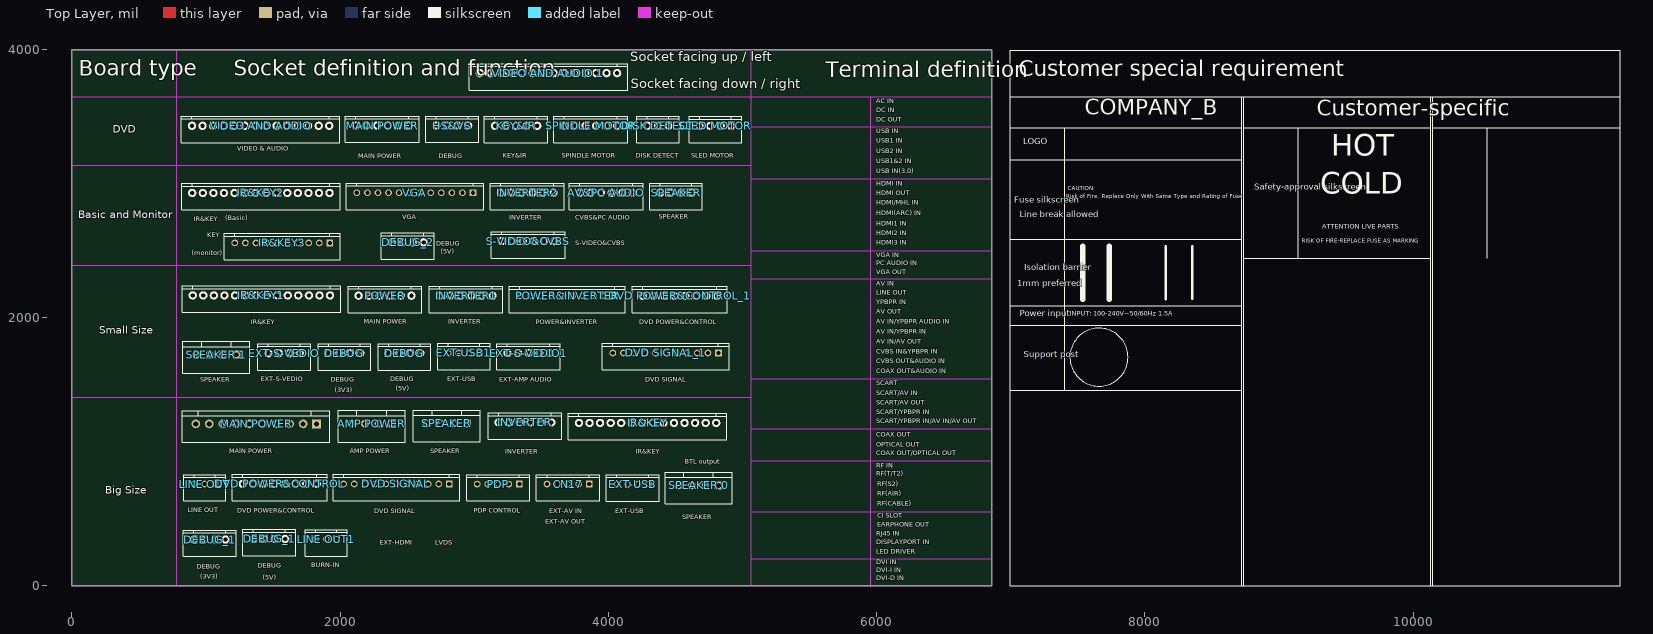
[diagram p0: Top Layer view]
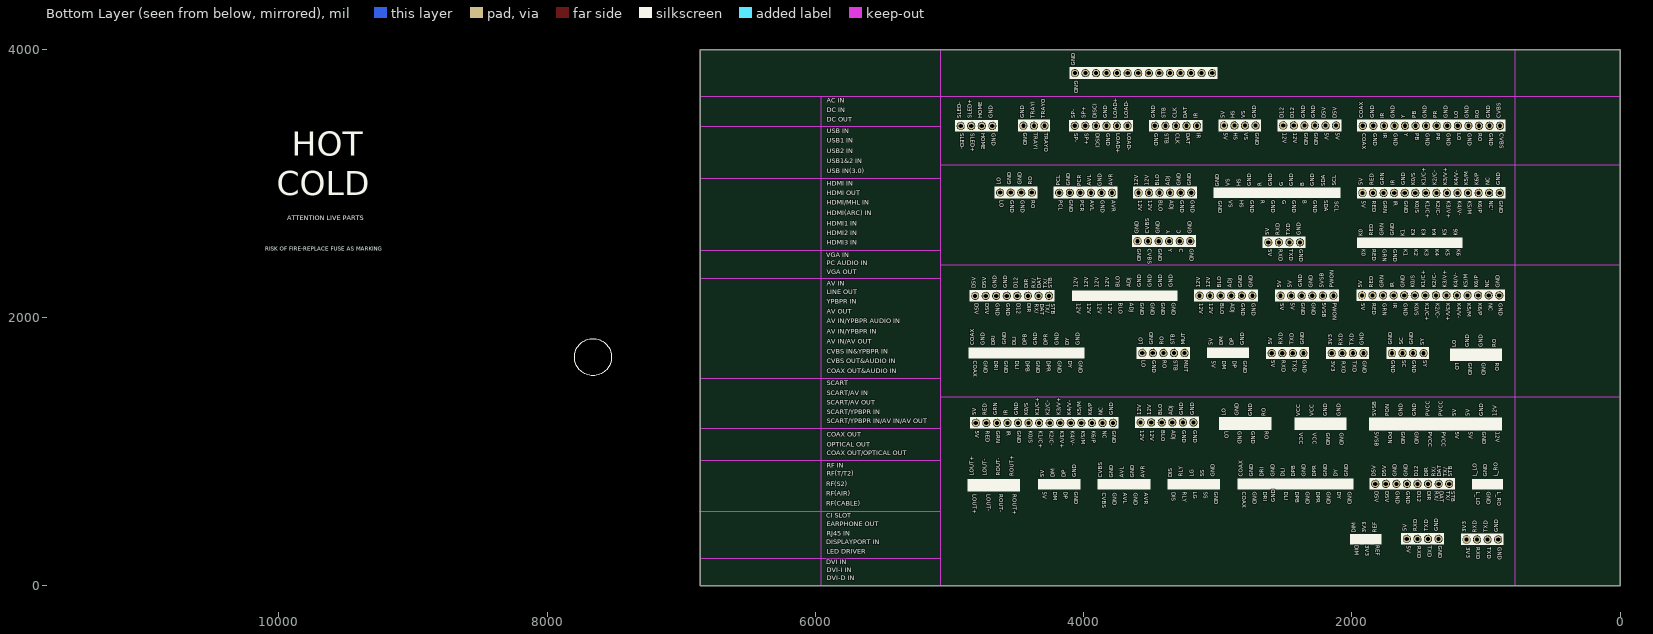
[diagram p1: Bottom Layer view, seen from below]
# Altium PCB MISC86383-7.PcbDoc
Units mil, origin at the board's own origin, x right, y up, seen from the top; angles counter-clockwise.
Board outline 6857.1 x 3995.31 mil, 2 copper layers (Top Layer, Bottom Layer); 43 components, 0 nets, 392 pads, 0 vias.

## Layer stack, top to bottom (the 12.6 mil dielectric is the usual default, probably not edited)
Top Solder: solder mask 0.4, Solder Resist, Dk 3.5
Top Layer: signal copper 1.4
Dielectric1: dielectric 12.6, FR-4, Dk 4.8
Bottom Layer: signal copper 1.4
Bottom Solder: solder mask 0.4, Solder Resist, Dk 3.5

## Board outline
0,0 0,3995.31 6857.1,3995.31 6857.1,0

## Design rules (kind name [scope] priority, off if disabled: settings)
Clearance [All] p1: gap=10 ignorepadtopadclearanceinfootprint=FALSE
PolygonConnect [All] p1: connectstyle=Relief reliefconductorwidth=10 reliefentries=4 polygonreliefangle="90 Angle" airgapwidth=10
RoutingVias [All] p1: holewidth=28 width=50 viastyle="Through Hole" minholewidth=28 minwidth=50 maxholewidth=28 maxwidth=50
SilkToSolderMaskClearance SilkscreenOverComponentPads [IsPad] p1: minsilkscreentomaskgap=10 clearancetoexposedcopper=TRUE
SolderMaskExpansion [All] p1: expansion=4 istentingtop=FALSE
Width [All] p1: maxlimit=10 minlimit=10 preferedwidth=10
29 further rules are at their usual default settings.

## Components (designator, comment, footprint, x,y, rotation, side; value= is the part's Value field where it differs from the comment)
"AMP POWER" "4PIN-2.54-D-H-red-G" SIP4/2.54DA 2235.61,1208.18 r0 top
"AV&PC AUDIO" "NC/6PIN-2.0-D-H-G" SIP6/2.0DA 3985.22,2930.06 r0 top
CN17 "5PIN-2.0-D-H-G" SIP5/2.0DA#1 3700.13,758.18 r0 top
DEBUG "4PIN-2.0-D-H-blue-G" SIP4/2.0DA#1 2031.99,1733.9 r0 top
DEBUG "4PIN-2.0-D-H-G" SIP4/2.0DA#1 2479.54,1733.9 r0 top
DEBUG_1 "4PIN-2.0-D-H-G" SIP4/2.0DA#1 1471.92,348.56 r0 top
DEBUG_1 "4PIN-2.0-D-H-blue-G" SIP4/2.0DA#1 1027.38,344.56 r0 top
DEBUG_2 "4PIN-2.0-D-H-G" SIP4/2.0DA#1 2504.72,2560.12 r0 top
"DISK DETECT" "3PIN-2.0-L-H-G" SIP3/2.0DA#1 4370.6,3430.3 r0 top
"DVD POWER&CONTROL" "6PIN-2.0-D-H-G" SIP8/2.0DA 1549.87,759.26 r0 top
"DVD POWER&CONTROL_1" "6PIN-2.0-D-H-G" SIP8/2.0DA 4533.96,2161.11 r0 top
"DVD SIGNAL" "11PIN-2.0-D-H-G" SIP11/2.0DA 2420.09,758.63 r0 top (schematic designator CN27)
"DVD SIGNAL_1" "11PIN-2.0-D-H-G" SIP11/2.0DA 4427.36,1735.49 r0 top (schematic designator CN27)
EXT-S-VEDIO "4PIN-2.0-D-H-G" SIP4/2.0DA#1 1583.02,1734.01 r0 top (schematic designator CN16)
EXT-S-VEDIO1 "4PIN-2.0-D-H-G" SIP5/2.0DA#2 3405.25,1734.69 r0 top (schematic designator CN16)
EXT-USB "NC/4PIN-2.0-D-H-G" SIP4/2.0DA#2 4182.24,755.94 r0 top
EXT-USB1 "NC/4PIN-2.0-D-H-G" SIP4/2.0DA#2 2923.57,1735.85 r0 top
HS&VS "4PIN-2.0-L-H-G" SIP4/2.0DA#1 2836.21,3431.3 r0 top
INVERTER "6PIN-2.0-D-H-G" SIP6/2.0DA 3378.32,1217.63 r0 top
INVERTER1 "6PIN-2.0-D-H-G" SIP6/2.0DA 2938.84,2162.9 r0 top
INVERTER2 "6PIN-2.0-D-H-G" SIP6/2.0DA 3394.56,2930.45 r0 top
IR&KEY "14PIN-2.0-D-H-G" SIP14/2.0DA 4292.78,1213.94 r0 top
IR&KEY1 "14PIN-2.0-D-H-G" SIP14/2.0DA 1412.75,2164.7 r0 top
IR&KEY2 "14PIN-2.0-D-H-G" SIP14/2.0DA 1409.16,2928.7 r0 top
IR&KEY3 "14PIN-2.0-D-H-G" SIP10/2.0DA 1569.17,2556.12 r0 top
KEY&IR "5PIN-2.0-L-H-G" SIP5/2.0DA#2 3311.72,3429.3 r0 top
"LINE OUT" "3PIN-2.0-D-H-G" SIP3/2.0DA#2 989.64,757.98 r0 top (schematic designator CN27)
"LINE OUT1" "3PIN-2.0-D-H-G" SIP3/2.0DA#2 1896.64,346.98 r0 top (schematic designator CN27)
"MAIN POWER" "6PIN-2.0-L-H-G" SIP6/2.0DA 2314.72,3431.3 r0 top
"MAIN POWER" "10PIN-2.54-D-H-G" SIP10/2.54DA 1373.86,1206.45 r0 top (schematic designator CN2)
PDP "NC/5PIN-2.0-D-H-G" SIP5/2.0DA#1 3179.18,757.74 r0 top (schematic designator CN4)
POWER "NC/4PIN-2.0-D-H-G" SIP6/2.0DA 2334.62,2162.9 r0 top
POWER&INVERTER "NC/6PIN-2.0-D-H-G" SIP10/2.0DA 3694.01,2161.12 r0 top
S-VIDEO&CVBS "NC/6PIN-2.0-D-H" SIP6/2.0DA 3401.5,2569.18 r0 top
"SLED MOTOR" "4PIN-2.0-L-H-G" SIP4/2.0DA#1 4798.94,3428.3 r0 top locked
SPEAKER "4PIN-2.54-D-H-G" SIP4/2.0DA#1 4504.61,2931.06 r0 top
SPEAKER "4PIN-2.54-D-H-G" SIP4/2.54DA 2796.61,1210.18 r0 top
"SPEAKER 0" "4PIN-2.54-D-H-G" SIP4/2.54DA 4672.61,748.18 r0 top
"SPEAKER 1" "4PIN-2.54-D-H-G" SIP4/2.54DA 1077.07,1723 r0 top
"SPINDLE MOTOR" "6PIN-2.0-L-H-G" SIP6/2.0DA 3869.48,3429.3 r0 top
VGA "NC/14PIN-2.0-D-H-G" SIP12/2.0DA 2557.81,2930.06 r0 top
"VIDEO AND AUDIO" "14PIN-2.0-L-H-G" SIP14/2.0DA 1406.97,3429.52 r0 top
"VIDEO AND AUDIO 1" "14PIN-2.0-L-H-G" SIP14/2.0DA 3553.61,3822.18 r0 top

## Footprints (in the part's own frame and the unit in brackets; to place one, negate y for a bottom-side part, rotate by r counter-clockwise, add the part's x,y. Pads: shape width x height; smd on the part's side, far side on the other; paste and mask are expansions set on the pad)
SIP3/2.0DA#1 [mm]
  oct 1.27x1.27 hole 0.8: 1(2,0)
  round 1.27 hole 0.8: 2(0,0) 3(-2,0)
  silkscreen extent -4,-3.2 4,1.8, body extent -4,-3.2 4,1.8, height 6
SIP3/2.0DA#2 [mm]
  rect 1.27x1.27 hole 0.8: 1(2,0)
  round 1.27 hole 0.8: 2(0,0) 3(-2,0)
  round 1.524 on Top Overlay: ""(-2,0) ""(0,0)
  rect 1.524x1.524 on Top Overlay: ""(2,0)
  silkscreen extent -4,-3.2 4,1.8, body extent -4,-3.2 4,1.8, height 6
SIP4/2.0DA#1 [mm]
  oct 1.27x1.27 hole 0.8: 1(3,0)
  round 1.27 hole 0.8: 2(1,0) 3(-1,0) 4(-3,0)
  silkscreen extent -5,-3.2 5,1.8, body extent -5,-3.2 5,1.8, height 6
SIP4/2.0DA#2 [mm]
  rect 1.27x1.27 hole 0.8: 1(3,0)
  round 1.27 hole 0.8: 2(1,0) 3(-1,0) 4(-3,0)
  round 1.524 on Top Overlay: ""(-3,0) ""(-1,0) ""(1,0)
  rect 1.524x1.524 on Top Overlay: ""(3,0)
  silkscreen extent -5,-3.2 5,1.8, body extent -5,-3.2 5,1.8, height 6
SIP4/2.54DA [mm]
  rect 1.5x1.5 hole 0.9: 1(3.81,0)
  round 1.5 hole 0.9: 2(1.27,0) 3(-1.27,0) 4(-3.81,0)
  round 1.8 on Top Overlay: ""(-3.81,0) ""(-1.27,0) ""(1.27,0)
  rect 1.8x1.8 on Top Overlay: ""(3.81,0)
  silkscreen extent -6.35,-3.5 6.35,2.5, body extent -6.35,-3.5 6.35,2.5, height 7
SIP5/2.0DA#1 [mm]
  rect 1.27x1.27 hole 0.8: 1(4,0)
  round 1.27 hole 0.8: 2(2,0) 3(0,0) 4(-2,0) 5(-4,0)
  round 1.524 on Top Overlay: ""(-4,0) ""(-2,0) ""(0,0) ""(2,0)
  rect 1.524x1.524 on Top Overlay: ""(4,0)
  silkscreen extent -6,-3.2 6,1.8, body extent -6,-3.2 6,1.8, height 6
SIP5/2.0DA#2 [mm]
  oct 1.27x1.27 hole 0.8: 1(4,0)
  round 1.27 hole 0.8: 2(2,0) 3(0,0) 4(-2,0) 5(-4,0)
  silkscreen extent -6,-3.2 6,1.8, body extent -6,-3.2 6,1.8, height 6
SIP6/2.0DA [mm]
  oct 1.27x1.27 hole 0.8: 1(5,0)
  round 1.27 hole 0.8: 2(3,0) 3(1,0) 4(-1,0) 5(-3,0) 6(-5,0)
  silkscreen extent -7,-3.2 7,1.8, body extent -7,-3.2 7,1.8, height 6
SIP8/2.0DA [mm]
  oct 1.27x1.27 hole 0.8: 1(7,0)
  round 1.27 hole 0.8: 2(5,0) 3(3,0) 4(1,0) 5(-1,0) 6(-3,0) 7(-5,0) 8(-7,0)
  silkscreen extent -9,-3.2 9,1.8, body extent -9,-3.2 9,1.8, height 6
SIP10/2.0DA [mm]
  rect 1.27x1.27 hole 0.8: 1(9,0)
  round 1.27 hole 0.8: 2(7,0) 3(5,0) 4(3,0) 5(1,0) 6(-1,0) 7(-3,0) 8(-5,0) 9(-7,0) 10(-9,0)
  round 1.524 on Top Overlay: ""(-9,0) ""(-7,0) ""(-5,0) ""(-3,0) ""(-1,0) ""(1,0) ""(3,0) ""(5,0) ""(7,0)
  rect 1.524x1.524 on Top Overlay: ""(9,0)
  silkscreen extent -11,-3.2 11,1.8, body extent -11,-3.2 11,1.8, height 6
SIP10/2.54DA [mil]
  rect 65x65 hole 39.37: 1(450,0)
  round 65 hole 39.37: 2(350,0) 3(250,0) 4(150,0) 5(50,0) 6(-50,0) 7(-150,0) 8(-250,0) 9(-350,0) 10(-450,0)
  round 75 on Top Overlay: ""(-450,0) ""(-350,0) ""(-250,0) ""(-150,0) ""(-50,0) ""(50,0) ""(150,0) ""(250,0) ""(350,0)
  rect 75x75 on Top Overlay: ""(450,0)
  silkscreen extent -550,-138 550,98, body extent -550,-138 550,98, height 276
SIP11/2.0DA [mm]
  rect 1.27x1.27 hole 0.8: 1(10,0)
  round 1.27 hole 0.8: 2(8,0) 3(6,0) 4(4,0) 5(2,0) 6(0,0) 7(-2,0) 8(-4,0) 9(-6,0) 10(-8,0) 11(-10,0)
  round 1.524 on Top Overlay: ""(-10,0) ""(-8,0) ""(-6,0) ""(-4,0) ""(-2,0) ""(0,0) ""(2,0) ""(4,0) ""(6,0) ""(8,0)
  rect 1.524x1.524 on Top Overlay: ""(10,0)
  silkscreen extent -12,-3.2 12,1.8, body extent -12,-3.2 12,1.8, height 6
SIP12/2.0DA [mm]
  rect 1.27x1.27 hole 0.8: 1(11,0)
  round 1.27 hole 0.8: 2(9,0) 3(7,0) 4(5,0) 5(3,0) 6(1,0) 7(-1,0) 8(-3,0) 9(-5,0) 10(-7,0) 11(-9,0) 12(-11,0)
  round 1.524 on Top Overlay: ""(-11,0) ""(-9,0) ""(-7,0) ""(-5,0) ""(-3,0) ""(-1,0) ""(1,0) ""(3,0) ""(5,0) ""(7,0) ""(9,0)
  rect 1.524x1.524 on Top Overlay: ""(11,0)
  silkscreen extent -13,-3.2 13,1.8, body extent -13,-3.2 13,1.8, height 6
SIP14/2.0DA [mm]
  oct 1.27x1.27 hole 0.8: 1(13,0)
  round 1.27 hole 0.8: 2(11,0) 3(9,0) 4(7,0) 5(5,0) 6(3,0) 7(1,0) 8(-1,0) 9(-3,0) 10(-5,0) 11(-7,0) 12(-9,0) 13(-11,0) 14(-13,0)
  silkscreen extent -15,-3.2 15,1.8, body extent -15,-3.2 15,1.8, height 6

## Part data
CN17 PDP: library part 5PIN
"DVD SIGNAL" "DVD SIGNAL_1": library part 11PIN
EXT-S-VEDIO EXT-S-VEDIO1 EXT-USB EXT-USB1: library part 4PIN
"LINE OUT" "LINE OUT1": library part CON3, "Connector"
"MAIN POWER": library part 10PIN

## Free pads (board coordinates)
  round 137.8 on Keep-Out: 0(7658.68,1704.32)

## Nets (pads, with @x,y where several pads share a name; then routed paths per layer and width w, separated by ;. In a path a pad name is that pad's centre, name@x,y a point inside that pad or via, vN(x,y) a via of type N, cw(c..) or ccw(c..) an arc to the next point about the centre after c; other vN are vias at no path point)
pads on no net: "AMP POWER.1" "AMP POWER.2" "AMP POWER.3" "AMP POWER.4" "AMP POWER." "AV&PC AUDIO.1" "AV&PC AUDIO.2" "AV&PC AUDIO.3" "AV&PC AUDIO.4" "AV&PC AUDIO.5" "AV&PC AUDIO.6" "DISK DETECT.1" "DISK DETECT.2" "DISK DETECT.3" "DVD POWER&CONTROL.1" "DVD POWER&CONTROL.2" "DVD POWER&CONTROL.3" "DVD POWER&CONTROL.4" "DVD POWER&CONTROL.5" "DVD POWER&CONTROL.6" "DVD POWER&CONTROL.7" "DVD POWER&CONTROL.8" "DVD POWER&CONTROL_1.1" "DVD POWER&CONTROL_1.2" "DVD POWER&CONTROL_1.3" "DVD POWER&CONTROL_1.4" "DVD POWER&CONTROL_1.5" "DVD POWER&CONTROL_1.6" "DVD POWER&CONTROL_1.7" "DVD POWER&CONTROL_1.8" "DVD SIGNAL.1" "DVD SIGNAL.2" "DVD SIGNAL.3" "DVD SIGNAL.4" "DVD SIGNAL.5" "DVD SIGNAL.6" "DVD SIGNAL.7" "DVD SIGNAL.8" "DVD SIGNAL.9" "DVD SIGNAL.10" "DVD SIGNAL.11" "DVD SIGNAL." "DVD SIGNAL_1.1" "DVD SIGNAL_1.2" "DVD SIGNAL_1.3" "DVD SIGNAL_1.4" "DVD SIGNAL_1.5" "DVD SIGNAL_1.6" "DVD SIGNAL_1.7" "DVD SIGNAL_1.8" "DVD SIGNAL_1.9" "DVD SIGNAL_1.10" "DVD SIGNAL_1.11" "DVD SIGNAL_1." "LINE OUT1.1" "LINE OUT1.2" "LINE OUT1.3" "LINE OUT1." "LINE OUT.1" "LINE OUT.2" "LINE OUT.3" "LINE OUT." "MAIN POWER.1" "MAIN POWER.2" "MAIN POWER.3" "MAIN POWER.4" "MAIN POWER.5" "MAIN POWER.6" "MAIN POWER.7" "MAIN POWER.8" "MAIN POWER.9" "MAIN POWER.10" "MAIN POWER." "SLED MOTOR.1" "SLED MOTOR.2" "SLED MOTOR.3" "SLED MOTOR.4" "SPEAKER 0.1" "SPEAKER 0.2" "SPEAKER 0.3" "SPEAKER 0.4" "SPEAKER 0." "SPEAKER 1.1" "SPEAKER 1.2" "SPEAKER 1.3" "SPEAKER 1.4" "SPEAKER 1." "SPINDLE MOTOR.1" "SPINDLE MOTOR.2" "SPINDLE MOTOR.3" "SPINDLE MOTOR.4" "SPINDLE MOTOR.5" "SPINDLE MOTOR.6" "VIDEO AND AUDIO 1.1" "VIDEO AND AUDIO 1.2" "VIDEO AND AUDIO 1.3" "VIDEO AND AUDIO 1.4" "VIDEO AND AUDIO 1.5" "VIDEO AND AUDIO 1.6" "VIDEO AND AUDIO 1.7" "VIDEO AND AUDIO 1.8" "VIDEO AND AUDIO 1.9" "VIDEO AND AUDIO 1.10" "VIDEO AND AUDIO 1.11" "VIDEO AND AUDIO 1.12" "VIDEO AND AUDIO 1.13" "VIDEO AND AUDIO 1.14" "VIDEO AND AUDIO.1" "VIDEO AND AUDIO.2" "VIDEO AND AUDIO.3" "VIDEO AND AUDIO.4" "VIDEO AND AUDIO.5" "VIDEO AND AUDIO.6" "VIDEO AND AUDIO.7" "VIDEO AND AUDIO.8" "VIDEO AND AUDIO.9" "VIDEO AND AUDIO.10" "VIDEO AND AUDIO.11" "VIDEO AND AUDIO.12" "VIDEO AND AUDIO.13" "VIDEO AND AUDIO.14" CN17. CN17.1 CN17.2 CN17.3 CN17.4 CN17.5 DEBUG.1 DEBUG.2 DEBUG.3 DEBUG.4 DEBUG_1.1 DEBUG_1.2 DEBUG_1.3 DEBUG_1.4 DEBUG_2.1 DEBUG_2.2 DEBUG_2.3 DEBUG_2.4 EXT-S-VEDIO1.1 EXT-S-VEDIO1.2 EXT-S-VEDIO1.3 EXT-S-VEDIO1.4 EXT-S-VEDIO1.5 EXT-S-VEDIO.1 EXT-S-VEDIO.2 EXT-S-VEDIO.3 EXT-S-VEDIO.4 EXT-USB1. EXT-USB1.1 EXT-USB1.2 EXT-USB1.3 EXT-USB1.4 EXT-USB. EXT-USB.1 EXT-USB.2 EXT-USB.3 EXT-USB.4 HS&VS.1 HS&VS.2 HS&VS.3 HS&VS.4 INVERTER1.1 INVERTER1.2 INVERTER1.3 INVERTER1.4 INVERTER1.5 INVERTER1.6 INVERTER2.1 INVERTER2.2 INVERTER2.3 INVERTER2.4 INVERTER2.5 INVERTER2.6 INVERTER.1 INVERTER.2 INVERTER.3 INVERTER.4 INVERTER.5 INVERTER.6 IR&KEY1.1 IR&KEY1.2 IR&KEY1.3 IR&KEY1.4 IR&KEY1.5 IR&KEY1.6 IR&KEY1.7 IR&KEY1.8 IR&KEY1.9 IR&KEY1.10 IR&KEY1.11 IR&KEY1.12 IR&KEY1.13 IR&KEY1.14 IR&KEY2.1 IR&KEY2.2 IR&KEY2.3 IR&KEY2.4 IR&KEY2.5 IR&KEY2.6 IR&KEY2.7 IR&KEY2.8 IR&KEY2.9 IR&KEY2.10 IR&KEY2.11 IR&KEY2.12 IR&KEY2.13 IR&KEY2.14 IR&KEY3. IR&KEY3.1 IR&KEY3.2 IR&KEY3.3 IR&KEY3.4 IR&KEY3.5 IR&KEY3.6 IR&KEY3.7 IR&KEY3.8 IR&KEY3.9 IR&KEY3.10 IR&KEY.1 IR&KEY.2 IR&KEY.3 IR&KEY.4 IR&KEY.5 IR&KEY.6 IR&KEY.7 IR&KEY.8 IR&KEY.9 IR&KEY.10 IR&KEY.11 IR&KEY.12 IR&KEY.13 IR&KEY.14 KEY&IR.1 KEY&IR.2 KEY&IR.3 KEY&IR.4 KEY&IR.5 PDP. PDP.1 PDP.2 PDP.3 PDP.4 PDP.5 POWER&INVERTER. POWER&INVERTER.1 POWER&INVERTER.2 POWER&INVERTER.3 POWER&INVERTER.4 POWER&INVERTER.5 POWER&INVERTER.6 POWER&INVERTER.7 POWER&INVERTER.8 POWER&INVERTER.9 POWER&INVERTER.10 POWER.1 POWER.2 POWER.3 POWER.4 POWER.5 POWER.6 S-VIDEO&CVBS.1 S-VIDEO&CVBS.2 S-VIDEO&CVBS.3 S-VIDEO&CVBS.4 S-VIDEO&CVBS.5 S-VIDEO&CVBS.6 SPEAKER. SPEAKER.1 SPEAKER.2 SPEAKER.3 SPEAKER.4 VGA. VGA.1 VGA.2 VGA.3 VGA.4 VGA.5 VGA.6 VGA.7 VGA.8 VGA.9 VGA.10 VGA.11 VGA.12

## Keep-outs
Keep-Out Layer:
  lines w4: 0,1406.21 5064.69,1406.21 ; 0,2387.82 5064.69,2387.82 ; 0,3133.82 5064.69,3133.82 ; 0,3647.6 6857.1,3647.6 ; 781.05,0 781.05,3995.31 ; 5064.69,202.18 6857.1,202.18 ; 5064.69,931.18 6857.1,931.18 ; 5064.69,1171.18 6857.1,1171.18 ; 5064.69,1543.18 6857.1,1543.18 ; 5064.69,2287.18 6857.1,2287.18 ; 5064.69,2499.18 6857.1,2499.18 ; 5064.69,3034.18 6857.1,3034.18 ; 5064.69,3423.18 6857.1,3423.18 ; 5064.69,3995.31 5064.69,0 ; 5074.69,553.18 6867.1,553.18 ; 5956.61,0 5956.61,3647.6 ; 5064.69,0 6857.1,0 6857.1,3995.31 0,3995.31 0,0 5064.69,0
  text "Update: 2017.02.23" at 0.61,4133.18 h300

## Silkscreen, mask and mechanical layers (free items; w line width, h text height)
Top Overlay:
  circle w5: c7658.68,1704.32 r216.54
  lines w5: 6998.1,1128.81 6998.1,3650.3 ; 6998.1,1456.28 8724.16,1456.28 ; 6998.1,1943.32 8724.16,1943.32 ; 6998.1,2086.91 8724.16,2086.91 ; 6998.1,2583.14 8724.16,2583.14 ; 6998.1,3175.81 8724.16,3175.81 ; 6998.1,3414.08 8724.16,3414.08 ; 6998.1,3647.6 8724.16,3647.6 ; 7404.91,1456.28 7404.91,3414.08 ; 8724.16,0 8724.16,1128.81 8724.16,3647.6 ; 8736.33,0 8736.33,3647.6 ; 8736.33,2443 10134.16,2443 ; 8736.33,3414 10134.16,3414.08 ; 9143.14,2443 9143.14,3414.08 ; 10134.16,0.08 10134.16,3647.6 ; 10146.33,0.08 10146.33,3647.6 ; 10146.33,3414 11544.16,3414.08 ; 10553.14,2443 10553.14,3414.08 ; 11544.16,3647.6 8724.16,3647.6 ; 6998.1,0 6998.1,3993.42 11544.16,3993.42 11544.16,0 6998.1,0
  lines w19.68: 8156.85,2138.38 8156.85,2531.38 ; 8353.7,2140.38 8353.7,2531.38
  lines w40: 7538.17,2136.96 7538.17,2532.38 ; 7735.02,2136.96 7735.02,2531.51
  text "Socket facing up / left" at 4161.61,3883.18 h120
  text "Socket definition and function" at 1207,3762 h200
  text "Board type" at 50.61,3761.18 h200
  text "Customer special requirement" at 7061,3757 h200
  text "Terminal definition" at 5621.61,3752.18 h200
  text "Socket facing down / right" at 4165.61,3682.18 h120
  text "AC IN" at 5996.61,3584.18 h60
  text "DC IN" at 5997.61,3514.18 h60
  text "COMPANY_B" at 7553.6,3470.8 h200
  text "Customer-specific" at 9281,3462 h200
  text "DC OUT" at 5997.61,3446.18 h60
  text "USB IN" at 5997.61,3357.18 h60
  text "DVD" at 304.61,3355.18 h100
  text "USB1 IN" at 5997.61,3288.18 h60
  text "LOGO" at 7093.67,3274.92 h78.74
  text "VIDEO & AUDIO" at 1234.61,3228.18 h60
  text "USB2 IN" at 5997.61,3210.18 h60
  text "SLED MOTOR" at 4616.61,3177.18 h60
  text "KEY&IR" at 3212.61,3176.18 h60
  text "SPINDLE MOTOR" at 3653.61,3176.18 h60
  text "DISK DETECT" at 4202.61,3176.18 h60
  text "DEBUG" at 2735.61,3174.18 h60
  text "MAIN POWER" at 2135.61,3173.18 h60
  text "HOT" at 9390.55,3148.71 h275.59
  text "USB1&2 IN" at 5997.61,3135.18 h60
  text "USB IN(3.0)" at 5997.61,3062.18 h60
  text "HDMI IN" at 5996.61,2966.18 h60
  text "CAUTION:" at 7427,2938 h50
  text "Safety-approval silkscreen" at 8815.16,2933 h78.74
  text "HDMI OUT" at 5996.61,2897.18 h60
  text "Risk of Fire, Replace Only With Same Type and Rating of Fuse" at 7413,2879 h50
  text "COLD" at 9307.02,2865.25 h275.59
  text "Fuse silkscreen" at 7027,2838 h78.74
  text "HDMI/MHL IN" at 5996.61,2824.18 h60
  text "HDMI(ARC) IN" at 5996.61,2749.18 h60
  text "Line break allowed" at 7068.52,2727.31 h78.74
  text "SPEAKER" at 4375.61,2720.18 h60
  text "VGA" at 2462.61,2718.18 h60
  text "Basic and Monitor" at 46.61,2717.18 h100
  text "INVERTER" at 3260.61,2715.18 h60
  text "CVBS&PC AUDIO" at 3753.61,2715.18 h60
  text "(Basic)" at 1142.61,2709.18 h60
  text "IR&KEY" at 907.61,2704.18 h60
  text "HDMI1 IN" at 5996.61,2670.18 h60
  text "ATTENTION LIVE PARTS" at 9322.01,2646.01 h59.06
  text "HDMI2 IN" at 5997.61,2600.18 h60
  text "KEY" at 1008.61,2584.18 h60
  text "RISK OF FIRE-REPLACE FUSE AS MARKING" at 9171.16,2548 h50
  text "HDMI3 IN" at 5996.61,2527.18 h60
  text "S-VIDEO&CVBS" at 3751.61,2525.18 h60
  text "DEBUG" at 2717.61,2519.18 h60
  text "(5V)" at 2750.61,2460.18 h60
  text "(monitor)" at 893.61,2450.18 h60
  text "VGA IN" at 5996.61,2436.18 h60
  text "PC AUDIO IN" at 5996.61,2374.18 h60
  text "Isolation barrier" at 7100,2334 h78.74
  text "VGA OUT" at 5996.61,2309.18 h60
  text "AV IN" at 5997.61,2222.18 h60
  text "1mm preferred" at 7050,2214 h78.74
  text "LINE OUT" at 5997.61,2156.18 h60
  text "YPBPR IN" at 5996.61,2085.18 h60
  text "AV OUT" at 5997.61,2011.18 h60
  text "INPUT:" at 7440.45,1998.43 h60
  text "100-240V~50/60Hz 1.5A" at 7617.46,1998.11 h60
  text "Power input" at 7068.6,1988.8 h78.74
  text "AV IN/YPBPR AUDIO IN" at 5996.61,1940.18 h60
  text "MAIN POWER" at 2176.61,1937.18 h60
  text "INVERTER" at 2806.61,1937.18 h60
  text "IR&KEY" at 1334.61,1935.18 h60
  text "POWER&INVERTER" at 3457.61,1935.18 h60
  text "DVD POWER&CONTROL" at 4230.61,1935.18 h60
  text "AV IN/YPBPR IN" at 5996.61,1865.18 h60
  text "Small Size" at 205.61,1855.18 h100
  text "AV IN/AV OUT" at 5997.61,1790.18 h60
  text "CVBS IN&YPBPR IN" at 5997.61,1714.18 h60
  text "Support post" at 7098,1686 h78.74
  text "CVBS OUT&AUDIO IN" at 5997.61,1644.18 h60
  text "COAX OUT&AUDIO IN" at 5996.61,1569.18 h60
  text "EXT-S-VEDIO" at 1409.61,1509.18 h60
  text "DEBUG" at 2374.61,1509.18 h60
  text "EXT-USB" at 2800.61,1509.18 h60
  text "SPEAKER" at 957.61,1507.18 h60
  text "DEBUG" at 1931.61,1507.18 h60
  text "EXT-AMP AUDIO" at 3185.61,1507.18 h60
  text "DVD SIGNAL" at 4273.61,1505.18 h60
  text "SCART" at 5998.61,1478.18 h60
  text "(5V)" at 2416.61,1439.18 h60
  text "(3V3)" at 1960.61,1429.18 h60
  text "SCART/AV IN" at 5997.61,1405.18 h60
  text "SCART/AV OUT" at 5996.61,1335.18 h60
  text "SCART/YPBPR IN" at 5996.61,1263.18 h60
  text "SCART/YPBPR IN/AV IN/AV OUT" at 5996.61,1196.18 h60
  text "COAX OUT" at 5996.61,1097.18 h60
  text "OPTICAL OUT" at 5996.61,1022.18 h60
  text "MAIN POWER" at 1171.61,973.18 h60
  text "AMP POWER" at 2071.61,971.18 h60
  text "SPEAKER" at 2671.61,971.18 h60
  text "INVERTER" at 3229.61,970.18 h60
  text "IR&KEY" at 4204.61,968.18 h60
  text "COAX OUT/OPTICAL OUT" at 5996.61,959.18 h60
  text "BTL output" at 4569.67,895.79 h60
  text "RF IN" at 5996.61,866.18 h60
  text "RF(T/T2)" at 5997.61,805.18 h60
  text "RF(S2)" at 6005.61,728.45 h60
  text "Big Size" at 247.61,662.18 h100
  text "RF(AIR)" at 6005.61,655.93 h60
  text "RF(CABLE)" at 6005.61,582.41 h60
  text "LINE OUT" at 864.61,531.18 h60
  text "DVD POWER&CONTROL" at 1234.61,529.18 h60
  text "PDP CONTROL" at 2996.61,529.18 h60
  text "DVD SIGNAL" at 2253.61,527.18 h60
  text "EXT-AV IN" at 3558.61,525.18 h60
  text "EXT-USB" at 4052.61,525.18 h60
  text "CI SLOT" at 6005.61,490.44 h60
  text "SPEAKER" at 4550.61,479.18 h60
  text "EXT-AV OUT" at 3528.61,446.18 h60
  text "EARPHONE OUT" at 6004.61,425.18 h60
  text "RJ45 IN" at 5997.61,358.18 h60
  text "DISPLAYPORT IN" at 5996.61,293.18 h60
  text "EXT-HDMI" at 2295.61,292.18 h60
  text "LVDS" at 2707.61,292.18 h60
  text "LED DRIVER" at 5997.61,223.18 h60
  text "DVI IN" at 5996.61,144.18 h60
  text "BURN-IN" at 1783.61,121.18 h60
  text "DEBUG" at 1384.61,118.18 h60
  text "DEBUG" at 930.61,113.18 h60
  text "DVI-I IN" at 5996.61,85.18 h60
  text "(3V3)" at 955.61,37.18 h60
  text "(5V)" at 1422.61,31.18 h60
  text "DVI-D IN" at 5996.61,24.18 h60
Bottom Overlay:
  circle w5: c7658.68,1704.32 r137.8
  text "GND" at 4051.32,3877.15 h50 r270
  text "GND" at 4081.32,3767.15 h50 r90
  text "AC IN" at 5915.61,3585.18 h60
  text "DC IN" at 5915.61,3514.18 h60
  text "D5V" at 2101.78,3487.15 h50 r270
  text "D5V" at 2182.95,3487.15 h50 r270
  text "GND" at 2261.62,3487.15 h50 r270
  text "GND" at 2337.79,3487.15 h50 r270
  text "D12" at 2418.96,3487.15 h50 r270
  text "D12" at 2496.38,3487.15 h50 r270
  text "GND" at 2703.18,3487.15 h50 r270
  text "VS" at 2782.53,3487.15 h50 r270
  text "HS" at 2861.88,3487.15 h50 r270
  text "5V" at 2938.26,3487.15 h50 r270
  text "TRAYO" at 4276.41,3486.15 h50 r270
  text "TRAYI" at 4354.62,3486.15 h50 r270
  text "GND" at 4432.83,3486.15 h50 r270
  text "CVBS" at 879.64,3485.15 h50 r270
  text "GND" at 958.17,3485.15 h50 r270
  text "RO" at 1037.49,3485.15 h50 r270
  text "GND" at 1116.82,3485.15 h50 r270
  text "LO" at 1194.54,3485.15 h50 r270
  text "GND" at 1273.01,3485.15 h50 r270
  text "PR" at 1352.14,3485.15 h50 r270
  text "GND" at 1430.84,3485.15 h50 r270
  text "PB" at 1509.54,3485.15 h50 r270
  text "Y" at 1589.21,3485.15 h50 r270
  text "GND" at 1668.39,3485.15 h50 r270
  text "IR" at 1745.64,3485.15 h50 r270
  text "GND" at 1823.38,3485.15 h50 r270
  text "COAX" at 1903.9,3485.15 h50 r270
  text "IR" at 3138.44,3485.15 h50 r270
  text "DAT" at 3217.32,3485.15 h50 r270
  text "CLK" at 3295.51,3485.15 h50 r270
  text "STB" at 3375.06,3485.15 h50 r270
  text "GND" at 3454.57,3485.15 h50 r270
  text "LOAD-" at 3657.41,3485.15 h50 r270
  text "LOAD+" at 3736.89,3485.15 h50 r270
  text "GND" at 3814.32,3485.15 h50 r270
  text "DISCI" at 3891.74,3485.15 h50 r270
  text "SP+" at 3972.25,3485.15 h50 r270
  text "SP-" at 4052.77,3485.15 h50 r270
  text "GND" at 4666.36,3484.15 h50 r270
  text "HOME" at 4743.97,3484.15 h50 r270
  text "SLED+" at 4823.37,3484.15 h50 r270
  text "SLED-" at 4901.58,3484.15 h50 r270
  text "DC OUT" at 5915.61,3446.18 h60
  text "5V" at 2131.78,3377.15 h50 r90
  text "5V" at 2212.95,3377.15 h50 r90
  text "GND" at 2291.62,3377.15 h50 r90
  text "GND" at 2367.79,3377.15 h50 r90
  text "12V" at 2448.96,3377.15 h50 r90
  text "12V" at 2526.38,3377.15 h50 r90
  text "GND" at 2733.18,3377.15 h50 r90
  text "VS" at 2812.53,3377.15 h50 r90
  text "HS" at 2891.88,3377.15 h50 r90
  text "5V" at 2968.26,3377.15 h50 r90
  text "TRAYO" at 4306.41,3376.15 h50 r90
  text "TRAYI" at 4384.62,3376.15 h50 r90
  text "GND" at 4462.83,3376.15 h50 r90
  text "CVBS" at 909.64,3375.15 h50 r90
  text "GND" at 988.17,3375.15 h50 r90
  text "RO" at 1067.49,3375.15 h50 r90
  text "GND" at 1146.82,3375.15 h50 r90
  text "LO" at 1224.54,3375.15 h50 r90
  text "GND" at 1303.01,3375.15 h50 r90
  text "PR" at 1382.14,3375.15 h50 r90
  text "GND" at 1460.84,3375.15 h50 r90
  text "PB" at 1539.54,3375.15 h50 r90
  text "Y" at 1619.21,3375.15 h50 r90
  text "GND" at 1698.39,3375.15 h50 r90
  text "IR" at 1775.64,3375.15 h50 r90
  text "GND" at 1853.38,3375.15 h50 r90
  text "COAX" at 1933.9,3375.15 h50 r90
  text "IR" at 3168.44,3375.15 h50 r90
  text "DAT" at 3247.32,3375.15 h50 r90
  text "CLK" at 3325.51,3375.15 h50 r90
  text "STB" at 3405.06,3375.15 h50 r90
  text "GND" at 3484.57,3375.15 h50 r90
  text "LOAD-" at 3687.41,3375.15 h50 r90
  text "LOAD+" at 3766.89,3375.15 h50 r90
  text "GND" at 3844.32,3375.15 h50 r90
  text "DISCI" at 3921.74,3375.15 h50 r90
  text "SP+" at 4002.25,3375.15 h50 r90
  text "SP-" at 4082.77,3375.15 h50 r90
  text "GND" at 4696.36,3374.15 h50 r90
  text "HOME" at 4773.97,3374.15 h50 r90
  text "SLED+" at 4853.37,3374.15 h50 r90
  text "SLED-" at 4931.58,3374.15 h50 r90
  text "USB IN" at 5916.61,3357.18 h60
  text "USB1 IN" at 5916.61,3288.18 h60
  text "USB2 IN" at 5915.61,3210.18 h60
  text "HOT" at 9906.29,3144.78 h307.09
  text "USB1&2 IN" at 5915.61,3135.18 h60
  text "USB IN(3.0)" at 5916.61,3062.18 h60
  text "RO" at 4372.04,2990.82 h50 r270
  text "GND" at 4449.62,2990.82 h50 r270
  text "GND" at 4528.55,2990.82 h50 r270
  text "LO" at 4606.13,2990.82 h50 r270
  text "GND" at 882.87,2987.05 h50 r270
  text "GND" at 1591.51,2987.05 h50 r270
  text "IR" at 1670.12,2987.05 h50 r270
  text "GRN" at 1748.04,2987.05 h50 r270
  text "RED" at 1827.46,2987.05 h50 r270
  text "5V" at 1907.64,2987.05 h50 r270
  text "NC" at 962.02,2986.18 h50 r270
  text "K6/P" at 1042.02,2986.18 h50 r270
  text "K5/M" at 1122.02,2986.18 h50 r270
  text "K4/V-" at 1197.02,2986.18 h50 r270
  text "K3/V+" at 1277.02,2986.18 h50 r270
  text "K2/C-" at 1357.02,2986.18 h50 r270
  text "K1/C+" at 1437.02,2986.18 h50 r270
  text "K0/S" at 1517.02,2986.18 h50 r270
  text "GND" at 3186.99,2983.8 h50 r270
  text "GND" at 3265.84,2983.8 h50 r270
  text "ADJ" at 3345.3,2983.8 h50 r270
  text "BLO" at 3424.77,2983.8 h50 r270
  text "12V" at 3504.23,2983.8 h50 r270
  text "12V" at 3580.2,2983.8 h50 r270
  text "SCL" at 2106.61,2983.18 h50 r270
  text "AVL" at 3933.61,2983.18 h50 r270
  text "GND" at 4089.22,2983.63 h50 r270
  text "PCL" at 4163.61,2983.18 h50 r270
  text "AVR" at 3772.1,2980.88 h50 r270
  text "SDA" at 2188.01,2979.82 h50 r270
  text "GND" at 2268.13,2979.82 h50 r270
  text "B" at 2345.7,2979.82 h50 r270
  text "GND" at 2425.18,2979.82 h50 r270
  text "G" at 2502.11,2979.82 h50 r270
  text "GND" at 2582.87,2979.82 h50 r270
  text "R" at 2661.72,2979.82 h50 r270
  text "GND" at 2739.28,2979.82 h50 r270
  text "HS" at 2818.13,2979.82 h50 r270
  text "VS" at 2899.54,2979.82 h50 r270
  text "GND" at 3853.09,2979.51 h50 r270
  text "PCR" at 4008.22,2979.51 h50 r270
  text "GND" at 2977.12,2976.26 h50 r270
  text "HDMI IN" at 5915.61,2967.18 h60
  text "HDMI OUT" at 5916.61,2898.18 h60
  text "GND" at 4119.22,2878.63 h50 r90
  text "AVR" at 3802.1,2875.88 h50 r90
  text "RO" at 4402.04,2875.82 h50 r90
  text "GND" at 4479.62,2875.82 h50 r90
  text "GND" at 4558.55,2875.82 h50 r90
  text "LO" at 4636.13,2875.82 h50 r90
  text "SDA" at 2218.01,2874.82 h50 r90
  text "GND" at 2298.13,2874.82 h50 r90
  text "B" at 2375.7,2874.82 h50 r90
  text "GND" at 2455.18,2874.82 h50 r90
  text "G" at 2532.11,2874.82 h50 r90
  text "GND" at 2612.87,2874.82 h50 r90
  text "R" at 2691.72,2874.82 h50 r90
  text "GND" at 2769.28,2874.82 h50 r90
  text "HS" at 2848.13,2874.82 h50 r90
  text "VS" at 2929.54,2874.82 h50 r90
  text "GND" at 3211.99,2873.8 h50 r90
  text "GND" at 3290.84,2873.8 h50 r90
  text "ADJ" at 3370.3,2873.8 h50 r90
  text "BLO" at 3449.77,2873.8 h50 r90
  text "12V" at 3529.23,2873.8 h50 r90
  text "12V" at 3605.2,2873.8 h50 r90
  text "GND" at 3883.09,2874.51 h50 r90
  text "PCR" at 4038.22,2874.51 h50 r90
  text "PCL" at 4196.1,2874.51 h50 r90
  text "AVL" at 3962.72,2873.14 h50 r90
  text "GND" at 912.87,2872.05 h50 r90
  text "GND" at 1621.51,2872.05 h50 r90
  text "IR" at 1700.12,2872.05 h50 r90
  text "GRN" at 1778.04,2872.05 h50 r90
  text "RED" at 1857.46,2872.05 h50 r90
  text "5V" at 1937.64,2872.05 h50 r90
  text "NC'" at 987.02,2871.18 h50 r90
  text "K6/P" at 1067.02,2871.18 h50 r90
  text "K5/M" at 1147.02,2871.18 h50 r90
  text "K4/V-" at 1222.02,2871.18 h50 r90
  text "K3/V+" at 1302.02,2871.18 h50 r90
  text "K2/C-" at 1382.02,2871.18 h50 r90
  text "K1/C+" at 1462.02,2871.18 h50 r90
  text "K0/S" at 1537.02,2871.18 h50 r90
  text "GND" at 3007.12,2871.26 h50 r90
  text "SCL" at 2139.16,2865.85 h50 r90
  text "COLD" at 10015.68,2853.44 h307.09
  text "HDMI/MHL IN" at 5915.61,2824.18 h60
  text "HDMI(ARC) IN" at 5915.61,2748.18 h60
  text "ATTENTION LIVE PARTS" at 9937.01,2711.01 h59.06
  text "HDMI1 IN" at 5915.61,2669.18 h60
  text "GND" at 3184.2,2623.94 h50 r270
  text "C" at 3263.53,2623.94 h50 r270
  text "Y" at 3344.37,2623.94 h50 r270
  text "GND" at 3421.72,2623.94 h50 r270
  text "CVBS" at 3500.01,2623.94 h50 r270
  text "GND" at 3578.3,2623.94 h50 r270
  text "GND" at 2370.97,2613.06 h50 r270
  text "TXD" at 2448.13,2613.06 h50 r270
  text "5V" at 2605.92,2613.06 h50 r270
  text "RXD" at 2527.89,2612.19 h50 r270
  text "K6" at 1201.04,2608.46 h50 r270
  text "K5" at 1280.53,2608.12 h50 r270
  text "K4" at 1359.02,2607.79 h50 r270
  text "K3" at 1437.18,2608.12 h50 r270
  text "K2" at 1516.34,2608.46 h50 r270
  text "GND" at 1673.34,2608.61 h50 r270
  text "GRN" at 1752.41,2607.94 h50 r270
  text "RED" at 1830.8,2607.94 h50 r270
  text "K1" at 1594.79,2607.65 h50 r270
  text "K0" at 1909.32,2607.29 h50 r270
  text "HDMI2 IN" at 5915.61,2600.18 h60
  text "HDMI3 IN" at 5916.61,2526.18 h60
  text "GND" at 3219.2,2513.94 h50 r90
  text "C" at 3298.53,2513.94 h50 r90
  text "Y" at 3379.37,2513.94 h50 r90
  text "GND" at 3456.72,2513.94 h50 r90
  text "CVBS" at 3535.01,2513.94 h50 r90
  text "GND" at 3613.3,2513.94 h50 r90
  text "GND" at 2404.61,2509.18 h50 r90
  text "K6" at 1231.04,2508.46 h50 r90
  text "K5" at 1310.53,2508.12 h50 r90
  text "K4" at 1389.02,2507.79 h50 r90
  text "K3" at 1467.18,2508.12 h50 r90
  text "K2" at 1546.34,2508.46 h50 r90
  text "GND" at 1703.34,2508.61 h50 r90
  text "GRN" at 1782.41,2507.94 h50 r90
  text "RED" at 1860.8,2507.94 h50 r90
  text "TXD" at 2478.13,2508.06 h50 r90
  text "5V" at 2635.92,2508.06 h50 r90
  text "K1" at 1624.79,2507.65 h50 r90
  text "K0" at 1939.32,2507.29 h50 r90
  text "RXD" at 2557.89,2507.19 h50 r90
  text "RISK OF FIRE-REPLACE FUSE AS MARKING" at 10103.16,2488 h50
  text "VGA IN" at 5917.61,2436.18 h60
  text "PC AUDIO IN" at 5915.61,2373.18 h60
  text "VGA OUT" at 5915.61,2309.18 h60
  text "GND" at 2359.37,2223.94 h50 r270
  text "GND" at 3323.19,2224.63 h50 r270
  text "GND" at 3402.41,2224.63 h50 r270
  text "GND" at 3481.99,2224.63 h50 r270
  text "GND" at 3561,2224.63 h50 r270
  text "ADJ" at 3638.6,2224.63 h50 r270
  text "BLO" at 3717.84,2224.63 h50 r270
  text "GND" at 886.46,2223.05 h50 r270
  text "GND" at 1595.1,2223.05 h50 r270
  text "IR" at 1673.71,2223.05 h50 r270
  text "GRN" at 1751.64,2223.05 h50 r270
  text "RED" at 1831.06,2223.05 h50 r270
  text "5V" at 1911.23,2223.05 h50 r270
  text "PWON" at 2123.32,2223.29 h50 r270
  text "5VSB" at 2200.28,2223.29 h50 r270
  text "GND" at 2280.47,2223.29 h50 r270
  text "5V" at 2437.63,2223.29 h50 r270
  text "AV IN" at 5915.61,2223.18 h60
  text "NC" at 965.61,2222.18 h50 r270
  text "K6/P" at 1045.61,2222.18 h50 r270
  text "K5/M" at 1125.61,2222.18 h50 r270
  text "K4/V-" at 1200.61,2222.18 h50 r270
  text "K3/V+" at 1280.61,2222.18 h50 r270
  text "K2/C-" at 1360.61,2222.18 h50 r270
  text "K1/C+" at 1440.61,2222.18 h50 r270
  text "K0/S" at 1520.61,2222.18 h50 r270
  text "5V" at 2515.23,2222.64 h50 r270
  text "12V" at 3796.92,2222.13 h50 r270
  text "12V" at 3876.01,2222.13 h50 r270
  text "12V" at 3953.54,2222.13 h50 r270
  text "12V" at 4032.63,2222.13 h50 r270
  text "GND" at 2726.26,2221.25 h50 r270
  text "GND" at 2805.12,2221.25 h50 r270
  text "ADJ" at 2884.58,2221.25 h50 r270
  text "BLO" at 2964.04,2221.25 h50 r270
  text "12V" at 3043.51,2221.25 h50 r270
  text "12V" at 3119.48,2221.25 h50 r270
  text "DIR" at 4402.16,2219.58 h50 r270
  text "D12" at 4479.61,2219.58 h50 r270
  text "GND" at 4557.98,2219.58 h50 r270
  text "GND" at 4636.49,2219.58 h50 r270
  text "D5V" at 4716.48,2219.58 h50 r270
  text "D5V" at 4794.44,2219.58 h50 r270
  text "DAT" at 4303.67,2218.58 h50 r270
  text "RX/" at 4347.17,2218.58 h50 r270
  text "STB" at 4224.48,2216.57 h50 r270
  text "TX/" at 4262.09,2216.57 h50 r270
  text "LINE OUT" at 5915.61,2157.18 h60
  text "GND" at 2389.37,2108.94 h50 r90
  text "GND" at 3353.19,2109.63 h50 r90
  text "GND" at 3432.41,2109.63 h50 r90
  text "GND" at 3511.99,2109.63 h50 r90
  text "GND" at 3591,2109.63 h50 r90
  text "ADJ" at 3668.6,2109.63 h50 r90
  text "BLO" at 3747.84,2109.63 h50 r90
  text "GND" at 916.46,2108.05 h50 r90
  text "GND" at 1625.1,2108.05 h50 r90
  text "IR" at 1703.71,2108.05 h50 r90
  text "GRN" at 1781.64,2108.05 h50 r90
  text "RED" at 1861.06,2108.05 h50 r90
  text "5V" at 1941.23,2108.05 h50 r90
  text "PWON" at 2153.32,2108.29 h50 r90
  text "5VSB" at 2230.28,2108.29 h50 r90
  text "GND" at 2310.47,2108.29 h50 r90
  text "5V" at 2467.63,2108.29 h50 r90
  text "NC" at 990.61,2107.18 h50 r90
  text "K6/P" at 1070.61,2107.18 h50 r90
  text "K5/M" at 1150.61,2107.18 h50 r90
  text "K4/V-" at 1225.61,2107.18 h50 r90
  text "K3/V+" at 1305.61,2107.18 h50 r90
  text "K2/C-" at 1385.61,2107.18 h50 r90
  text "K1/C+" at 1465.61,2107.18 h50 r90
  text "K0/S" at 1540.61,2107.18 h50 r90
  text "5V" at 2545.23,2107.64 h50 r90
  text "12V" at 3826.92,2107.13 h50 r90
  text "12V" at 3906.01,2107.13 h50 r90
  text "12V" at 3983.54,2107.13 h50 r90
  text "12V" at 4062.63,2107.13 h50 r90
  text "GND" at 2756.26,2106.25 h50 r90
  text "GND" at 2835.12,2106.25 h50 r90
  text "ADJ" at 2914.58,2106.25 h50 r90
  text "BLO" at 2994.04,2106.25 h50 r90
  text "12V" at 3073.51,2106.25 h50 r90
  text "12V" at 3149.48,2106.25 h50 r90
  text "DIR" at 4432.16,2104.58 h50 r90
  text "D12" at 4509.61,2104.58 h50 r90
  text "GND" at 4587.98,2104.58 h50 r90
  text "GND" at 4666.49,2104.58 h50 r90
  text "D5V" at 4746.48,2104.58 h50 r90
  text "D5V" at 4824.44,2104.58 h50 r90
  text "DAT" at 4333.67,2103.58 h50 r90
  text "RX/" at 4377.17,2103.58 h50 r90
  text "STB" at 4254.48,2101.57 h50 r90
  text "TX/" at 4292.09,2101.57 h50 r90
  text "YPBPR IN" at 5916.61,2086.18 h60
  text "AV OUT" at 5916.61,2011.18 h60
  text "AV IN/YPBPR AUDIO IN" at 5915.61,1941.18 h60
  text "AV IN/YPBPR IN" at 5915.61,1865.18 h60
  text "GND" at 2345.79,1796.84 h50 r270
  text "TXD" at 2422.95,1796.84 h50 r270
  text "5V" at 2580.74,1796.84 h50 r270
  text "GND" at 3470.81,1797 h50 r270
  text "SC" at 1606.81,1795.85 h50 r270
  text "RXD" at 2502.71,1795.97 h50 r270
  text "MUT" at 3231.37,1795.97 h50 r270
  text "STB" at 3310.93,1795.97 h50 r270
  text "RO" at 3392.03,1795.97 h50 r270
  text "LO" at 3546.75,1795.97 h50 r270
  text "GND" at 4566.61,1796.18 h50 r270
  text "GND" at 1529.65,1794.93 h50 r270
  text "GND" at 1686.51,1795.09 h50 r270
  text "SY" at 1448.84,1794.48 h50 r270
  text "GND" at 2790.91,1794.19 h50 r270
  text "DP" at 2869.56,1794.19 h50 r270
  text "DM" at 2949.01,1794.19 h50 r270
  text "5V" at 3027.4,1794.19 h50 r270
  text "GND" at 4018.51,1793.93 h50 r270
  text "DY" at 4096.92,1793.93 h50 r270
  text "GND" at 4175.82,1793.93 h50 r270
  text "DPR" at 4255.21,1793.93 h50 r270
  text "GND" at 4334.11,1793.93 h50 r270
  text "DPB" at 4412.37,1793.93 h50 r270
  text "DLI" at 4490.89,1793.93 h50 r270
  text "DRI" at 4648.18,1793.93 h50 r270
  text "GND" at 4727.32,1793.93 h50 r270
  text "COAX" at 4806.02,1793.93 h50 r270
  text "GND" at 1898.62,1792.18 h50 r270
  text "3V3" at 2134.63,1792.13 h50 r270
  text "TXD" at 1976.45,1791.32 h50 r270
  text "RXD" at 2057.71,1790.47 h50 r270
  text "AV IN/AV OUT" at 5916.61,1790.18 h60
  text "RO" at 912.8,1777.79 h50 r270
  text "GND" at 1012.74,1777.79 h50 r270
  text "GND" at 1112.68,1778.6 h50 r270
  text "LO" at 1211,1778.6 h50 r270
  text "CVBS IN&YPBPR IN" at 5915.61,1714.18 h60
  text "GND" at 2375.79,1681.84 h50 r90
  text "TXD" at 2452.95,1681.84 h50 r90
  text "5V" at 2610.74,1681.84 h50 r90
  text "GND" at 3500.81,1682 h50 r90
  text "SC" at 1636.81,1680.85 h50 r90
  text "RXD" at 2532.71,1680.97 h50 r90
  text "MUT" at 3261.37,1680.97 h50 r90
  text "STB" at 3340.93,1680.97 h50 r90
  text "RO" at 3422.03,1680.97 h50 r90
  text "LO" at 3576.75,1680.97 h50 r90
  text "GND" at 1559.65,1679.93 h50 r90
  text "GND" at 1716.51,1680.09 h50 r90
  text "SY" at 1478.84,1679.48 h50 r90
  text "GND" at 2820.91,1679.19 h50 r90
  text "DP" at 2899.56,1679.19 h50 r90
  text "DM" at 2979.01,1679.19 h50 r90
  text "5V" at 3057.4,1679.19 h50 r90
  text "GND" at 4048.51,1678.93 h50 r90
  text "DY" at 4126.92,1678.93 h50 r90
  text "GND" at 4205.82,1678.93 h50 r90
  text "DPR" at 4285.21,1678.93 h50 r90
  text "GND" at 4364.11,1678.93 h50 r90
  text "DPB" at 4442.37,1678.93 h50 r90
  text "DLI" at 4520.89,1678.93 h50 r90
  text "DRI" at 4678.18,1678.93 h50 r90
  text "GND" at 4757.32,1678.93 h50 r90
  text "COAX" at 4836.02,1678.93 h50 r90
  text "GND" at 1928.62,1677.18 h50 r90
  text "3V3" at 2164.63,1677.13 h50 r90
  text "TXD" at 2006.45,1676.32 h50 r90
  text "GND" at 4601.61,1676.18 h50 r90
  text "RXD" at 2087.71,1675.47 h50 r90
  text "RO" at 942.8,1662.79 h50 r90
  text "GND" at 1042.74,1662.79 h50 r90
  text "GND" at 1142.68,1663.6 h50 r90
  text "LO" at 1241,1663.6 h50 r90
  text "CVBS OUT&AUDIO IN" at 5915.61,1644.18 h60
  text "COAX OUT&AUDIO IN" at 5915.61,1570.18 h60
  text "SCART" at 5915.61,1478.18 h60
  text "SCART/AV IN" at 5916.61,1406.18 h60
  text "SCART/AV OUT" at 5916.61,1336.18 h60
  text "GND" at 3766.49,1272.29 h50 r270
  text "GND" at 4475.12,1272.29 h50 r270
  text "IR" at 4553.74,1272.29 h50 r270
  text "GRN" at 4631.66,1272.29 h50 r270
  text "RED" at 4711.08,1272.29 h50 r270
  text "5V" at 4791.26,1272.29 h50 r270
  text "GND" at 3165.74,1270.97 h50 r270
  text "GND" at 3244.59,1270.97 h50 r270
  text "ADJ" at 3324.05,1270.97 h50 r270
  text "BLO" at 3403.52,1270.97 h50 r270
  text "12V" at 3482.98,1270.97 h50 r270
  text "12V" at 3558.96,1270.97 h50 r270
  text "NC" at 3845.64,1271.42 h50 r270
  text "K6/P" at 3925.64,1271.42 h50 r270
  text "K5/M" at 4005.64,1271.42 h50 r270
  text "K4/V-" at 4080.64,1271.42 h50 r270
  text "K3/V+" at 4160.64,1271.42 h50 r270
  text "K2/C-" at 4240.64,1271.42 h50 r270
  text "K1/C+" at 4320.64,1271.42 h50 r270
  text "K0/S" at 4400.64,1271.42 h50 r270
  text "GND" at 2832.23,1265.77 h50 r270
  text "LO" at 2930.55,1265.77 h50 r270
  text "RO" at 2632.35,1264.96 h50 r270
  text "GND" at 2732.29,1264.96 h50 r270
  text "GND" at 2072.36,1264.02 h50 r270
  text "GND" at 2172.55,1264.02 h50 r270
  text "VCC" at 2273.46,1264.02 h50 r270
  text "VCC" at 2375.08,1264.02 h50 r270
  text "12V" at 907.09,1263.16 h50 r270
  text "GND" at 1008.01,1263.16 h50 r270
  text "5V" at 1108.58,1263.16 h50 r270
  text "5V" at 1209.15,1263.16 h50 r270
  text "PVCC" at 1309.36,1263.16 h50 r270
  text "PVCC" at 1409.22,1263.16 h50 r270
  text "GND" at 1508.37,1263.16 h50 r270
  text "GND" at 1609.29,1263.16 h50 r270
  text "PON" at 1708.79,1263.16 h50 r270
  text "5VSB" at 1808.3,1263.16 h50 r270
  text "SCART/YPBPR IN" at 5916.61,1263.18 h60
  text "SCART/YPBPR IN/AV IN/AV OUT" at 5916.61,1196.18 h60
  text "GND" at 3195.74,1160.97 h50 r90
  text "GND" at 3274.59,1160.97 h50 r90
  text "ADJ" at 3354.05,1160.97 h50 r90
  text "BLO" at 3433.52,1160.97 h50 r90
  text "12V" at 3512.98,1160.97 h50 r90
  text "12V" at 3588.96,1160.97 h50 r90
  text "GND" at 3796.49,1157.29 h50 r90
  text "GND" at 4505.12,1157.29 h50 r90
  text "IR" at 4583.74,1157.29 h50 r90
  text "GRN" at 4661.66,1157.29 h50 r90
  text "RED" at 4741.08,1157.29 h50 r90
  text "5V" at 4821.26,1157.29 h50 r90
  text "NC" at 3870.64,1156.42 h50 r90
  text "K6/P" at 3950.64,1156.42 h50 r90
  text "K5/M" at 4030.64,1156.42 h50 r90
  text "K4/V-" at 4105.64,1156.42 h50 r90
  text "K3/V+" at 4185.64,1156.42 h50 r90
  text "K2/C-" at 4265.64,1156.42 h50 r90
  text "K1/C+" at 4345.64,1156.42 h50 r90
  text "K0/S" at 4420.64,1156.42 h50 r90
  text "GND" at 2862.23,1150.77 h50 r90
  text "LO" at 2960.55,1150.77 h50 r90
  text "RO" at 2662.35,1149.96 h50 r90
  text "GND" at 2762.29,1149.96 h50 r90
  text "12V" at 939.34,1146.43 h50 r90
  text "GND" at 1040.26,1146.43 h50 r90
  text "5V" at 1140.83,1146.43 h50 r90
  text "5V" at 1241.39,1146.43 h50 r90
  text "PVCC" at 1341.61,1146.43 h50 r90
  text "PVCC" at 1441.46,1146.43 h50 r90
  text "GND" at 1540.62,1146.43 h50 r90
  text "GND" at 1641.54,1146.43 h50 r90
  text "PON" at 1741.04,1146.43 h50 r90
  text "5VSB" at 1840.54,1146.43 h50 r90
  text "GND" at 2102.36,1139.02 h50 r90
  text "GND" at 2202.55,1139.02 h50 r90
  text "VCC" at 2303.46,1139.02 h50 r90
  text "VCC" at 2405.08,1139.02 h50 r90
  text "COAX OUT" at 5916.61,1097.18 h60
  text "OPTICAL OUT" at 5916.61,1022.18 h60
  text "COAX OUT/OPTICAL OUT" at 5916.61,959.18 h60
  text "RF IN" at 5915.61,865.18 h60
  text "LOUT-" at 4709.63,819.73 h50 r270
  text "LOUT+" at 4807.94,819.73 h50 r270
  text "ROUT+" at 4509.22,817.96 h50 r270
  text "ROUT-" at 4609.26,818.48 h50 r270
  text "STB" at 1239.32,813.58 h50 r270
  text "TX/" at 1276.93,813.58 h50 r270
  text "DAT" at 1324.22,813.1 h50 r270
  text "RX/" at 1362.56,813.15 h50 r270
  text "DIR" at 1418.07,812.72 h50 r270
  text "D12" at 1495.53,812.72 h50 r270
  text "GND" at 1573.89,812.72 h50 r270
  text "GND" at 1652.41,812.72 h50 r270
  text "D5V" at 1732.39,812.72 h50 r270
  text "D5V" at 1810.36,812.72 h50 r270
  text "GND" at 2565.61,813.18 h50 r270
  text "GND" at 2016.23,812.08 h50 r270
  text "DY" at 2094.65,812.08 h50 r270
  text "GND" at 2173.55,812.08 h50 r270
  text "DPR" at 2252.93,812.08 h50 r270
  text "GND" at 2331.83,812.08 h50 r270
  text "DPB" at 2410.1,812.08 h50 r270
  text "DLI" at 2488.61,812.08 h50 r270
  text "DRI" at 2645.91,812.08 h50 r270
  text "GND" at 2725.05,812.08 h50 r270
  text "COAX" at 2803.74,812.08 h50 r270
  text "L_RO" at 900.85,810.72 h50 r270
  text "GND" at 979.39,810.72 h50 r270
  text "L_LO" at 1058.58,810.72 h50 r270
  text "GND" at 3010.7,811.09 h50 r270
  text "SS" at 3089.54,811.09 h50 r270
  text "LG" at 3168.79,811.09 h50 r270
  text "RLY" at 3248.46,811.09 h50 r270
  text "GND" at 4044.58,809.29 h50 r270
  text "DP" at 4123.23,809.29 h50 r270
  text "DM" at 4202.68,809.29 h50 r270
  text "5V" at 4281.06,809.29 h50 r270
  text "DIS" at 3328.1,808.57 h50 r270
  text "RF(T/T2)" at 5916.61,805.18 h60
  text "AVR" at 3533.53,803.49 h50 r270
  text "GND" at 3612.27,803.49 h50 r270
  text "AVL" at 3691.01,803.49 h50 r270
  text "GND" at 3769.75,803.49 h50 r270
  text "CVBS" at 3848.49,803.49 h50 r270
  text "RF(S2)" at 5917.61,728.45 h60
  text "STB" at 1269.32,703.58 h50 r90
  text "TX/" at 1306.93,703.58 h50 r90
  text "DAT" at 1354.22,703.1 h50 r90
  text "RX/" at 1392.56,703.15 h50 r90
  text "DIR" at 1448.07,702.72 h50 r90
  text "D12" at 1525.53,702.72 h50 r90
  text "GND" at 1603.89,702.72 h50 r90
  text "GND" at 1682.41,702.72 h50 r90
  text "D5V" at 1762.39,702.72 h50 r90
  text "D5V" at 1840.36,702.72 h50 r90
  text "GND" at 2041.23,702.08 h50 r90
  text "DY" at 2119.65,702.08 h50 r90
  text "GND" at 2198.55,702.08 h50 r90
  text "DPR" at 2277.93,702.08 h50 r90
  text "GND" at 2356.83,702.08 h50 r90
  text "DPB" at 2435.1,702.08 h50 r90
  text "DLI" at 2513.61,702.08 h50 r90
  text "DRI" at 2670.91,702.08 h50 r90
  text "GND" at 2750.05,702.08 h50 r90
  text "COAX" at 2828.74,702.08 h50 r90
  text "L_RO" at 925.85,700.72 h50 r90
  text "GND" at 1004.39,700.72 h50 r90
  text "L_LO" at 1083.58,700.72 h50 r90
  text "GND" at 3035.7,701.09 h50 r90
  text "SS" at 3114.54,701.09 h50 r90
  text "LG" at 3193.79,701.09 h50 r90
  text "RLY" at 3273.46,701.09 h50 r90
  text "GND" at 4079.58,699.29 h50 r90
  text "DP" at 4158.23,699.29 h50 r90
  text "DM" at 4237.68,699.29 h50 r90
  text "5V" at 4316.06,699.29 h50 r90
  text "DIS" at 3353.1,698.57 h50 r90
  text "AVR" at 3558.53,693.49 h50 r90
  text "GND" at 3637.27,693.49 h50 r90
  text "AVL" at 3716.01,693.49 h50 r90
  text "GND" at 3794.75,693.49 h50 r90
  text "CVBS" at 3873.49,693.49 h50 r90
  text "ROUT+" at 4539.67,680.79 h50 r90
  text "ROUT-" at 4639.67,680.79 h50 r90
  text "LOUT-" at 4734.67,680.79 h50 r90
  text "LOUT+" at 4839.67,680.79 h50 r90
  text "RF(AIR)" at 5917.61,655.93 h60
  text "GND" at 2561.1,620.96 h50 r270
  text "RF(CABLE)" at 5917.61,582.41 h60
  text "CI SLOT" at 5917.61,490.44 h60
  text "EARPHONE OUT" at 5915.61,427.18 h60
  text "GND" at 1343.18,406.5 h50 r270
  text "TXD" at 1420.34,406.5 h50 r270
  text "5V" at 1578.12,406.5 h50 r270
  text "RXD" at 1500.09,405.63 h50 r270
  text "GND" at 899,397.84 h50 r270
  text "3V3" at 1135.01,397.79 h50 r270
  text "TXD" at 976.83,396.99 h50 r270
  text "RXD" at 1058.09,396.13 h50 r270
  text "REF" at 1802.61,394.18 h50 r270
  text "3V3" at 1880.61,394.18 h50 r270
  text "DIM" at 1960.61,394.18 h50 r270
  text "RJ45 IN" at 5915.61,359.18 h60
  text "3V3" at 1912.61,302.18 h50 r90
  text "REF" at 1832.61,301.18 h50 r90
  text "DIM" at 1989.61,301.18 h50 r90
  text "GND" at 1368.18,296.5 h50 r90
  text "TXD" at 1445.34,296.5 h50 r90
  text "5V" at 1603.12,296.5 h50 r90
  text "RXD" at 1525.09,295.63 h50 r90
  text "DISPLAYPORT IN" at 5917.61,293.18 h60
  text "GND" at 924,287.84 h50 r90
  text "3V3" at 1160.01,287.79 h50 r90
  text "TXD" at 1001.83,286.99 h50 r90
  text "RXD" at 1083.09,286.13 h50 r90
  text "LED DRIVER" at 5915.61,224.18 h60
  text "DVI IN" at 5917.61,144.18 h60
  text "DVI-I IN" at 5916.61,84.18 h60
  text "DVI-D IN" at 5916.61,24.18 h60
  text "GND" at 3571.61,-1044.82 h59.06 r90
  text "GND" at 3491.61,-1046.82 h59.06 r90
  text "ADJ" at 3656.61,-1051.82 h59.06 r90
  text "12V" at 3810.61,-1051.82 h59.06 r90
  text "BLO" at 3728.61,-1052.82 h59.06 r90
  text "12V" at 3890.61,-1055.82 h59.06 r90